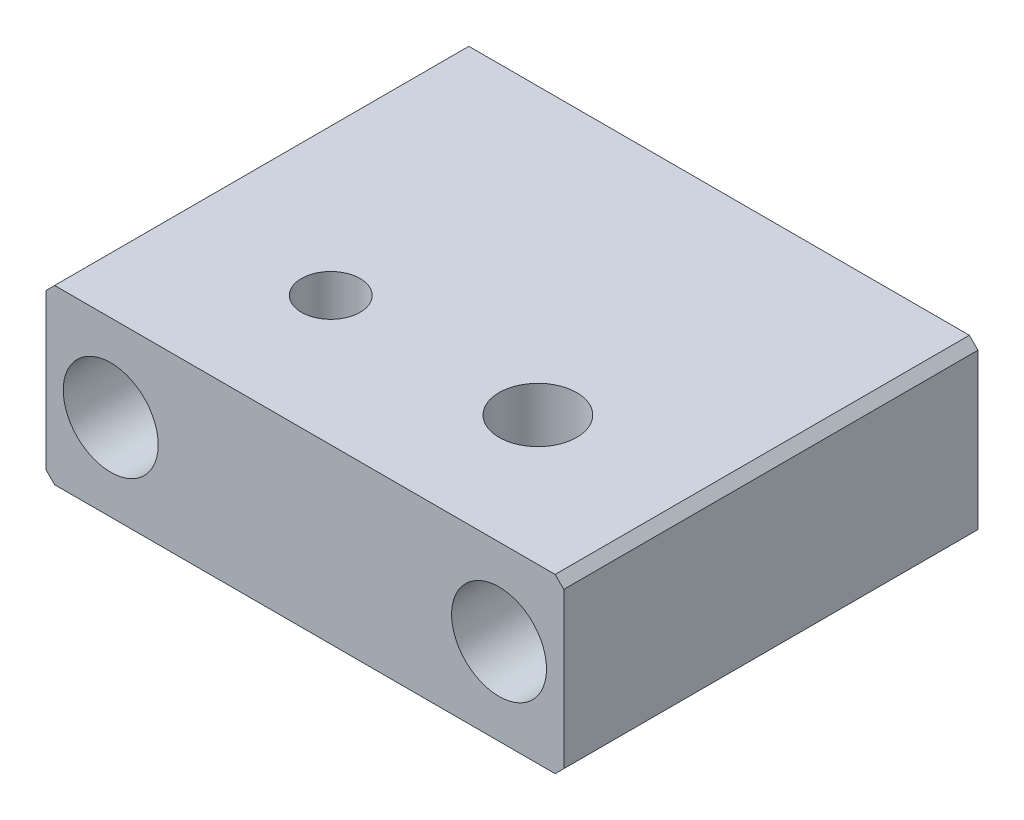
from build123d import *

# Parameters (mm, degrees)
SKETCH1_W                                           = 60
SKETCH1_H                                           = 20
BOSS_EXTRUDE1_DEPTH                                 = 48
CBORE_FOR_M6_HEX_SOCKET_HEAD_CAP_SCREW1_D           = 6.6
CBORE_FOR_M6_HEX_SOCKET_HEAD_CAP_SCREW1_CBORE_D     = 11
CBORE_FOR_M6_HEX_SOCKET_HEAD_CAP_SCREW1_CBORE_DEPTH = 8
M8_TAPPED_HOLE1_D                                   = 6.8
M10X1_0_TAPPED_HOLE1_D                              = 9
CHAMFER1_SIZE                                       = 1


with BuildPart() as part:
    # Sketch1 → Boss-Extrude1 (new body)
    with BuildSketch(Plane.XY):
        Rectangle(SKETCH1_W, SKETCH1_H)
    extrude(amount=BOSS_EXTRUDE1_DEPTH)

    # CBORE for M6 Hex Socket Head Cap Screw1 (through all)
    with Locations(Plane.XY.offset(48)):
        with Locations((-22.5, 0), (22.5, 0)):
            CounterBoreHole(CBORE_FOR_M6_HEX_SOCKET_HEAD_CAP_SCREW1_D / 2, CBORE_FOR_M6_HEX_SOCKET_HEAD_CAP_SCREW1_CBORE_D / 2, CBORE_FOR_M6_HEX_SOCKET_HEAD_CAP_SCREW1_CBORE_DEPTH)

    # M8 Tapped Hole1 (through all)
    with Locations(Plane.XZ.offset(10)):
        with Locations((-12, 33)):
            Hole(M8_TAPPED_HOLE1_D / 2)

    # M10x1.0 Tapped Hole1 (through all)
    with Locations(Plane.XZ.offset(10)):
        with Locations((12, 33)):
            Hole(M10X1_0_TAPPED_HOLE1_D / 2)

    # Chamfer1
    chamfer1_edges = [part.edges().sort_by_distance(p)[0] for p in [
        (30, -10, 24),
        (-30, -10, 24),
        (-30, 10, 24),
        (30, 10, 24),
    ]]
    chamfer(chamfer1_edges, length=CHAMFER1_SIZE)


solid = part.part
